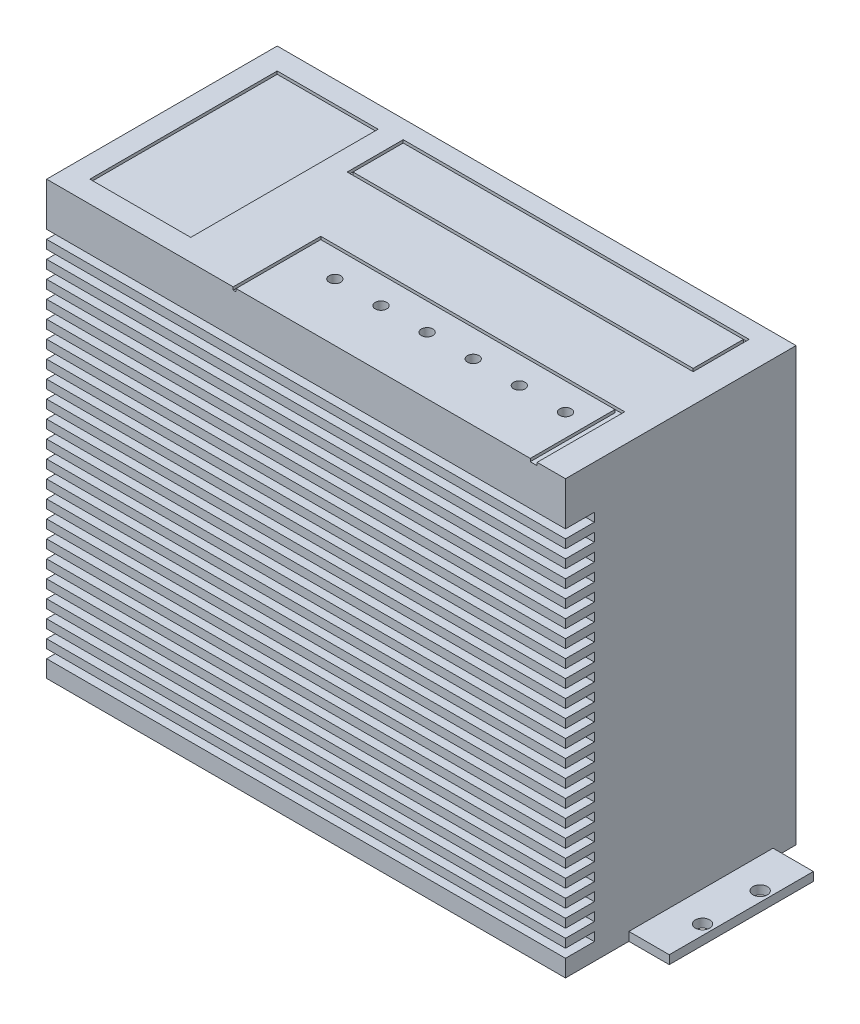
SolidWorks part; units mm, degrees
ref_plane "前视基准面" through (0, 0, 0) normal (0, 0, 1) x (1, 0, 0)
ref_plane "上视基准面" through (0, 0, 0) normal (0, 1, 0) x (1, 0, 0)
ref_plane "右视基准面" through (0, 0, 0) normal (1, 0, 0) x (0, 0, -1)
sketch "草图1" plane through (0, 0, 0) normal (0, 0, 1) x (1, 0, 0)
  line L1 (90, -75) -> (-90, -75)
  line L2 (90, -75) -> (90, 75)
  line L3 (90, 75) -> (-90, 75)
  line L4 (-90, -75) -> (-90, 75)
  line L5 (90, -75) -> (-90, 75) construction
  line L6 (90, 75) -> (-90, -75) construction
  point P0 (0, 0)
  dimension "D1" = 150
  dimension "D2" = 180
extrude "凸台-拉伸1" add sketch "草图1" along normal mid plane 80
sketch "草图2" plane through (-90, 0, 0) normal (-1, 0, 0) x (0, 0, 1)
  line L0 (40, 59.9231) -> (30, 59.9231)
  line L1 (40, 75) -> (40, -75) construction
  line L2 (30, 59.9231) -> (30, 56.9231)
  line L3 (30, 56.9231) -> (40, 56.9231)
  line L4 (40, 56.9231) -> (40, 59.9231)
  line L5 (40, 53.9231) -> (30, 53.9231)
  line L6 (30, 53.9231) -> (30, 50.9231)
  line L7 (40, 50.9231) -> (40, 53.9231)
  line L8 (30, 50.9231) -> (40, 50.9231)
  line L9 (40, 47.9231) -> (30, 47.9231)
  line L10 (30, 47.9231) -> (30, 44.9231)
  line L11 (40, 44.9231) -> (40, 47.9231)
  line L12 (30, 44.9231) -> (40, 44.9231)
  line L13 (40, 41.9231) -> (30, 41.9231)
  line L14 (30, 41.9231) -> (30, 38.9231)
  line L15 (40, 38.9231) -> (40, 41.9231)
  line L16 (30, 38.9231) -> (40, 38.9231)
  line L17 (40, 35.9231) -> (30, 35.9231)
  line L18 (30, 35.9231) -> (30, 32.9231)
  line L19 (40, 32.9231) -> (40, 35.9231)
  line L20 (30, 32.9231) -> (40, 32.9231)
  line L21 (40, 29.9231) -> (30, 29.9231)
  line L22 (30, 29.9231) -> (30, 26.9231)
  line L23 (40, 26.9231) -> (40, 29.9231)
  line L24 (30, 26.9231) -> (40, 26.9231)
  line L25 (40, 23.9231) -> (30, 23.9231)
  line L26 (30, 23.9231) -> (30, 20.9231)
  line L27 (40, 20.9231) -> (40, 23.9231)
  line L28 (30, 20.9231) -> (40, 20.9231)
  line L29 (40, 17.9231) -> (30, 17.9231)
  line L30 (30, 17.9231) -> (30, 14.9231)
  line L31 (40, 14.9231) -> (40, 17.9231)
  line L32 (30, 14.9231) -> (40, 14.9231)
  line L33 (40, 11.9231) -> (30, 11.9231)
  line L34 (30, 11.9231) -> (30, 8.9231)
  line L35 (40, 8.9231) -> (40, 11.9231)
  line L36 (30, 8.9231) -> (40, 8.9231)
  line L37 (40, 5.9231) -> (30, 5.9231)
  line L38 (30, 5.9231) -> (30, 2.9231)
  line L39 (40, 2.9231) -> (40, 5.9231)
  line L40 (30, 2.9231) -> (40, 2.9231)
  line L41 (40, -0.0769) -> (30, -0.0769)
  line L42 (30, -0.0769) -> (30, -3.0769)
  line L43 (40, -3.0769) -> (40, -0.0769)
  line L44 (30, -3.0769) -> (40, -3.0769)
  line L45 (40, -6.0769) -> (30, -6.0769)
  line L46 (30, -6.0769) -> (30, -9.0769)
  line L47 (40, -9.0769) -> (40, -6.0769)
  line L48 (30, -9.0769) -> (40, -9.0769)
  line L49 (40, -12.0769) -> (30, -12.0769)
  line L50 (30, -12.0769) -> (30, -15.0769)
  line L51 (40, -15.0769) -> (40, -12.0769)
  line L52 (30, -15.0769) -> (40, -15.0769)
  line L53 (40, -18.0769) -> (30, -18.0769)
  line L54 (30, -18.0769) -> (30, -21.0769)
  line L55 (40, -21.0769) -> (40, -18.0769)
  line L56 (30, -21.0769) -> (40, -21.0769)
  line L57 (40, -24.0769) -> (30, -24.0769)
  line L58 (30, -24.0769) -> (30, -27.0769)
  line L59 (40, -27.0769) -> (40, -24.0769)
  line L60 (30, -27.0769) -> (40, -27.0769)
  line L61 (40, -30.0769) -> (30, -30.0769)
  line L62 (30, -30.0769) -> (30, -33.0769)
  line L63 (40, -33.0769) -> (40, -30.0769)
  line L64 (30, -33.0769) -> (40, -33.0769)
  line L65 (40, -36.0769) -> (30, -36.0769)
  line L66 (30, -36.0769) -> (30, -39.0769)
  line L67 (40, -39.0769) -> (40, -36.0769)
  line L68 (30, -39.0769) -> (40, -39.0769)
  line L69 (40, -42.0769) -> (30, -42.0769)
  line L70 (30, -42.0769) -> (30, -45.0769)
  line L71 (40, -45.0769) -> (40, -42.0769)
  line L72 (30, -45.0769) -> (40, -45.0769)
  line L73 (40, -48.0769) -> (30, -48.0769)
  line L74 (30, -48.0769) -> (30, -51.0769)
  line L75 (40, -51.0769) -> (40, -48.0769)
  line L76 (30, -51.0769) -> (40, -51.0769)
  line L77 (40, -54.0769) -> (30, -54.0769)
  line L78 (30, -54.0769) -> (30, -57.0769)
  line L79 (40, -57.0769) -> (40, -54.0769)
  line L80 (30, -57.0769) -> (40, -57.0769)
  line L81 (40, -60.0769) -> (30, -60.0769)
  line L82 (30, -60.0769) -> (30, -63.0769)
  line L83 (40, -63.0769) -> (40, -60.0769)
  line L84 (30, -63.0769) -> (40, -63.0769)
  line L85 (40, -66.0769) -> (30, -66.0769)
  line L86 (30, -66.0769) -> (30, -69.0769)
  line L87 (40, -69.0769) -> (40, -66.0769)
  line L88 (30, -69.0769) -> (40, -69.0769)
  dimension "D1" = 10
  dimension "D2" = 3
  dimension "D3" = 22
extrude "切除-拉伸1" cut sketch "草图2" against normal up to next
sketch "草图3" plane through (0, 75, 0) normal (0, 1, 0) x (1, 0, 0)
  line L0 (-90, -40) -> (-90, 40) construction
  line L1 (-47.5, -32.5) -> (-82.5, -32.5)
  line L2 (-47.5, -32.5) -> (-47.5, 32.5)
  line L3 (-47.5, 32.5) -> (-82.5, 32.5)
  line L4 (-82.5, -32.5) -> (-82.5, 32.5)
  line L5 (-47.5, -32.5) -> (-82.5, 32.5) construction
  line L6 (-47.5, 32.5) -> (-82.5, -32.5) construction
  point P0 (-65, 0)
  dimension "D1" = 25
  dimension "D2" = 65
  dimension "D3" = 35
extrude "切除-拉伸2" cut sketch "草图3" against normal blind 1
sketch "草图4" plane through (0, 75, 0) normal (0, 1, 0) x (1, 0, 0)
  line L0 (90, 40) -> (-90, 40) construction
  line L1 (80, 14.2871) -> (-40, 14.2871)
  line L2 (80, 14.2871) -> (80, 33.7129)
  line L3 (80, 33.7129) -> (-40, 33.7129)
  line L4 (-40, 14.2871) -> (-40, 33.7129)
  line L5 (80, 14.2871) -> (-40, 33.7129) construction
  line L6 (80, 33.7129) -> (-40, 14.2871) construction
  line L8 (90, -40) -> (90, 40) construction
  line L10 (79, 15.2871) -> (-39, 15.2871)
  line L11 (79, 15.2871) -> (79, 32.7129)
  line L12 (79, 32.7129) -> (-39, 32.7129)
  line L13 (-39, 15.2871) -> (-39, 32.7129)
  line L14 (79, 15.2871) -> (-39, 32.7129) construction
  line L15 (79, 32.7129) -> (-39, 15.2871) construction
  point P0 (20, 24)
  point P9 (20, 24)
  dimension "D1" = 16
  dimension "D2" = 70
  dimension "D3" = 1
  dimension "D4" = 1
  dimension "D5" = 120
extrude "切除-拉伸3" cut sketch "草图4" against normal blind 1
sketch "草图5" plane through (0, -75, 0) normal (0, -1, 0) x (1, 0, 0)
  line L0 (-90, 40) -> (-90, -40) construction
  line L1 (-90, 18) -> (-104, 18)
  line L2 (-90, 18) -> (-90, -32)
  line L3 (-90, -32) -> (-104, -32)
  line L4 (-104, 18) -> (-104, -32)
  line L5 (-18.117, 0) -> (27.0821, 0) construction
  line L6 (0, 46.7867) -> (0, -21.7591) construction
  line L7 (-104, -7) -> (-84.8465, -7) construction
  line L8 (90, 18) -> (90, -32)
  line L9 (90, -32) -> (104, -32)
  line L10 (104, 18) -> (104, -32)
  line L11 (90, 18) -> (104, 18)
  circle A0 centre (-100.541, 3) radius 2.5
  circle A1 centre (-100.541, -17) radius 2.5
  circle A2 centre (100.541, 3) radius 2.5
  circle A3 centre (100.541, -17) radius 2.5
  dimension "D4" = 5
  dimension "D5" = 20
  dimension "D1" = 14
  dimension "D2" = 50
  dimension "D3" = 8
extrude "凸台-拉伸2" add sketch "草图5" against normal blind 3
sketch "草图6" plane through (0, 75, 0) normal (0, 1, 0) x (1, 0, 0)
  line L0 (90, -40) -> (-90, -40) construction
  line L2 (-90, -40) -> (-90, 40) construction
  circle A0 centre (-10, -20) radius 2
  circle A1 centre (6, -20) radius 2
  circle A2 centre (22, -20) radius 2
  circle A3 centre (38, -20) radius 2
  circle A4 centre (54, -20) radius 2
  circle A5 centre (70, -20) radius 2
  dimension "D1" = 4
  dimension "D2" = 20
  dimension "D4" = 80
  dimension "D3" = 6
extrude "切除-拉伸4" cut sketch "草图6" against normal blind 4
sketch "草图7" plane through (0, 75, 0) normal (0, 1, 0) x (1, 0, 0)
  line L0 (90, -40) -> (-90, -40) construction
  line L1 (-25.2795, -9.6148) -> (80.1596, -9.6148)
  line L2 (-25.2795, -9.6148) -> (-25.2795, -40)
  line L3 (-25.2795, -40) -> (80.1596, -40)
  line L4 (80.1596, -9.6148) -> (80.1596, -40)
  line L6 (-24.2795, -10.6148) -> (77.7829, -10.6148)
  line L7 (-24.2795, -10.6148) -> (-24.2795, -40)
  line L8 (-24.2795, -40) -> (77.7829, -40)
  line L9 (77.7829, -10.6148) -> (77.7829, -40)
  line M21 (-90, -40) -> (90, -40)
  dimension "D1" = 1
  dimension "D2" = 1
extrude "切除-拉伸5" cut sketch "草图7" against normal blind 1 contours L6 L9 L4 L1 L2 L7 M21
